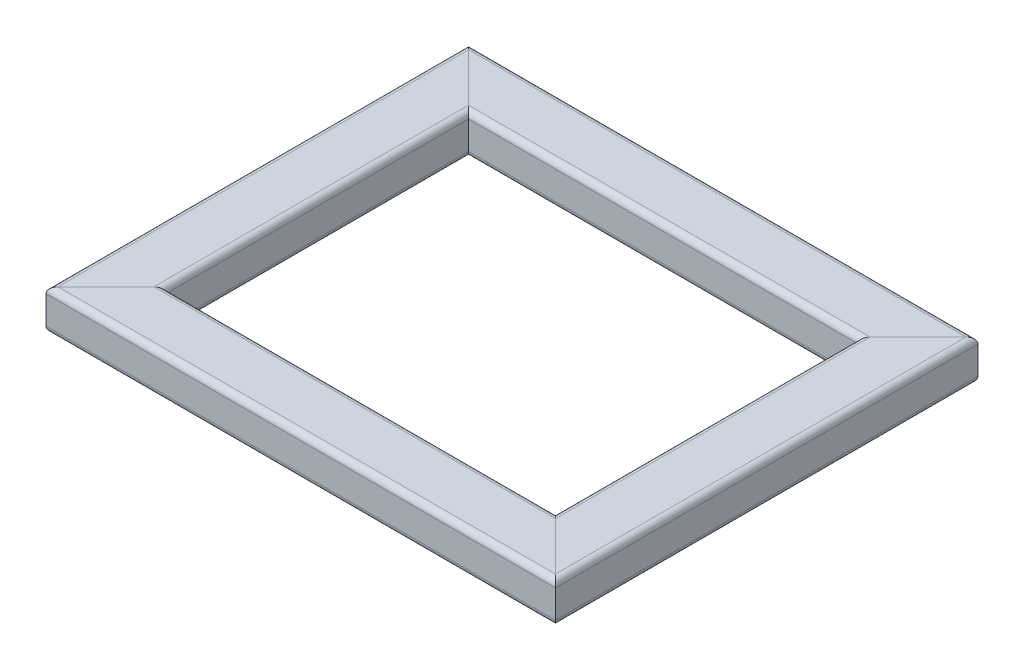
SolidWorks part; units mm, degrees
material "Q235B"
ref_plane "Front Plane" through (0, 0, 0) normal (0, 0, 1) x (1, 0, 0)
ref_plane "Top Plane" through (0, 0, 0) normal (0, 1, 0) x (1, 0, 0)
ref_plane "Right Plane" through (0, 0, 0) normal (1, 0, 0) x (0, 0, -1)
sketch "草图1" plane through (0, 0, 0) normal (0, 1, 0) x (1, 0, 0)
  line L1 (225, -181.5) -> (-225, -181.5)
  line L2 (225, -181.5) -> (225, 181.5)
  line L3 (225, 181.5) -> (-225, 181.5)
  line L4 (-225, -181.5) -> (-225, 181.5)
  line L5 (225, -181.5) -> (-225, 181.5) construction
  line L6 (225, 181.5) -> (-225, -181.5) construction
  point P0 (0, 0)
  dimension "D1" = 450
  dimension "D2" = 363
other "GB/T 6728-2002 Rectangular Hollow Section 60X40X3(1)"
ref_plane "Plane1" through (-225, 0, 181.5) normal (0, 0, -1) x (0, 1, 0)
sketch "Sketch1" plane through (-225, 0, 181.5) normal (0, 0, -1) x (0, 1, 0)
  line L0 (-14, -27) -> (14, -27)
  line L1 (-17, -24) -> (-17, 24)
  line L2 (14, 27) -> (-14, 27)
  line L3 (17, 24) -> (17, -24)
  line L4 (-14, -30) -> (14, -30)
  line L5 (-20, -24) -> (-20, 24)
  line L6 (14, 30) -> (-14, 30)
  line L7 (20, 24) -> (20, -24)
  arc A0 (20, 24) -> (14, 30) centre (14, 24) ccw
  arc A1 (14, -30) -> (20, -24) centre (14, -24) ccw
  arc A2 (-20, -24) -> (-14, -30) centre (-14, -24) ccw
  arc A3 (-14, 30) -> (-20, 24) centre (-14, 24) ccw
  arc A4 (-14, 27) -> (-17, 24) centre (-14, 24) ccw
  arc A5 (17, 24) -> (14, 27) centre (14, 24) ccw
  arc A6 (14, -27) -> (17, -24) centre (14, -24) ccw
  arc A7 (-17, -24) -> (-14, -27) centre (-14, -24) ccw
  point P0 (0, 30)
  point P1 (20, 0)
  point P2 (0, -30)
  point P3 (-20, 0)
  point P4 (-20, 30)
  point P5 (20, 30)
  point P6 (20, -30)
  point P7 (-20, -30)
  point P8 (0, 0)
  point P33 (0, 0)
  dimension "D1" = 6
  dimension "Thickness" = 3
  dimension "V_leg" = 60
  dimension "H_leg" = 40
